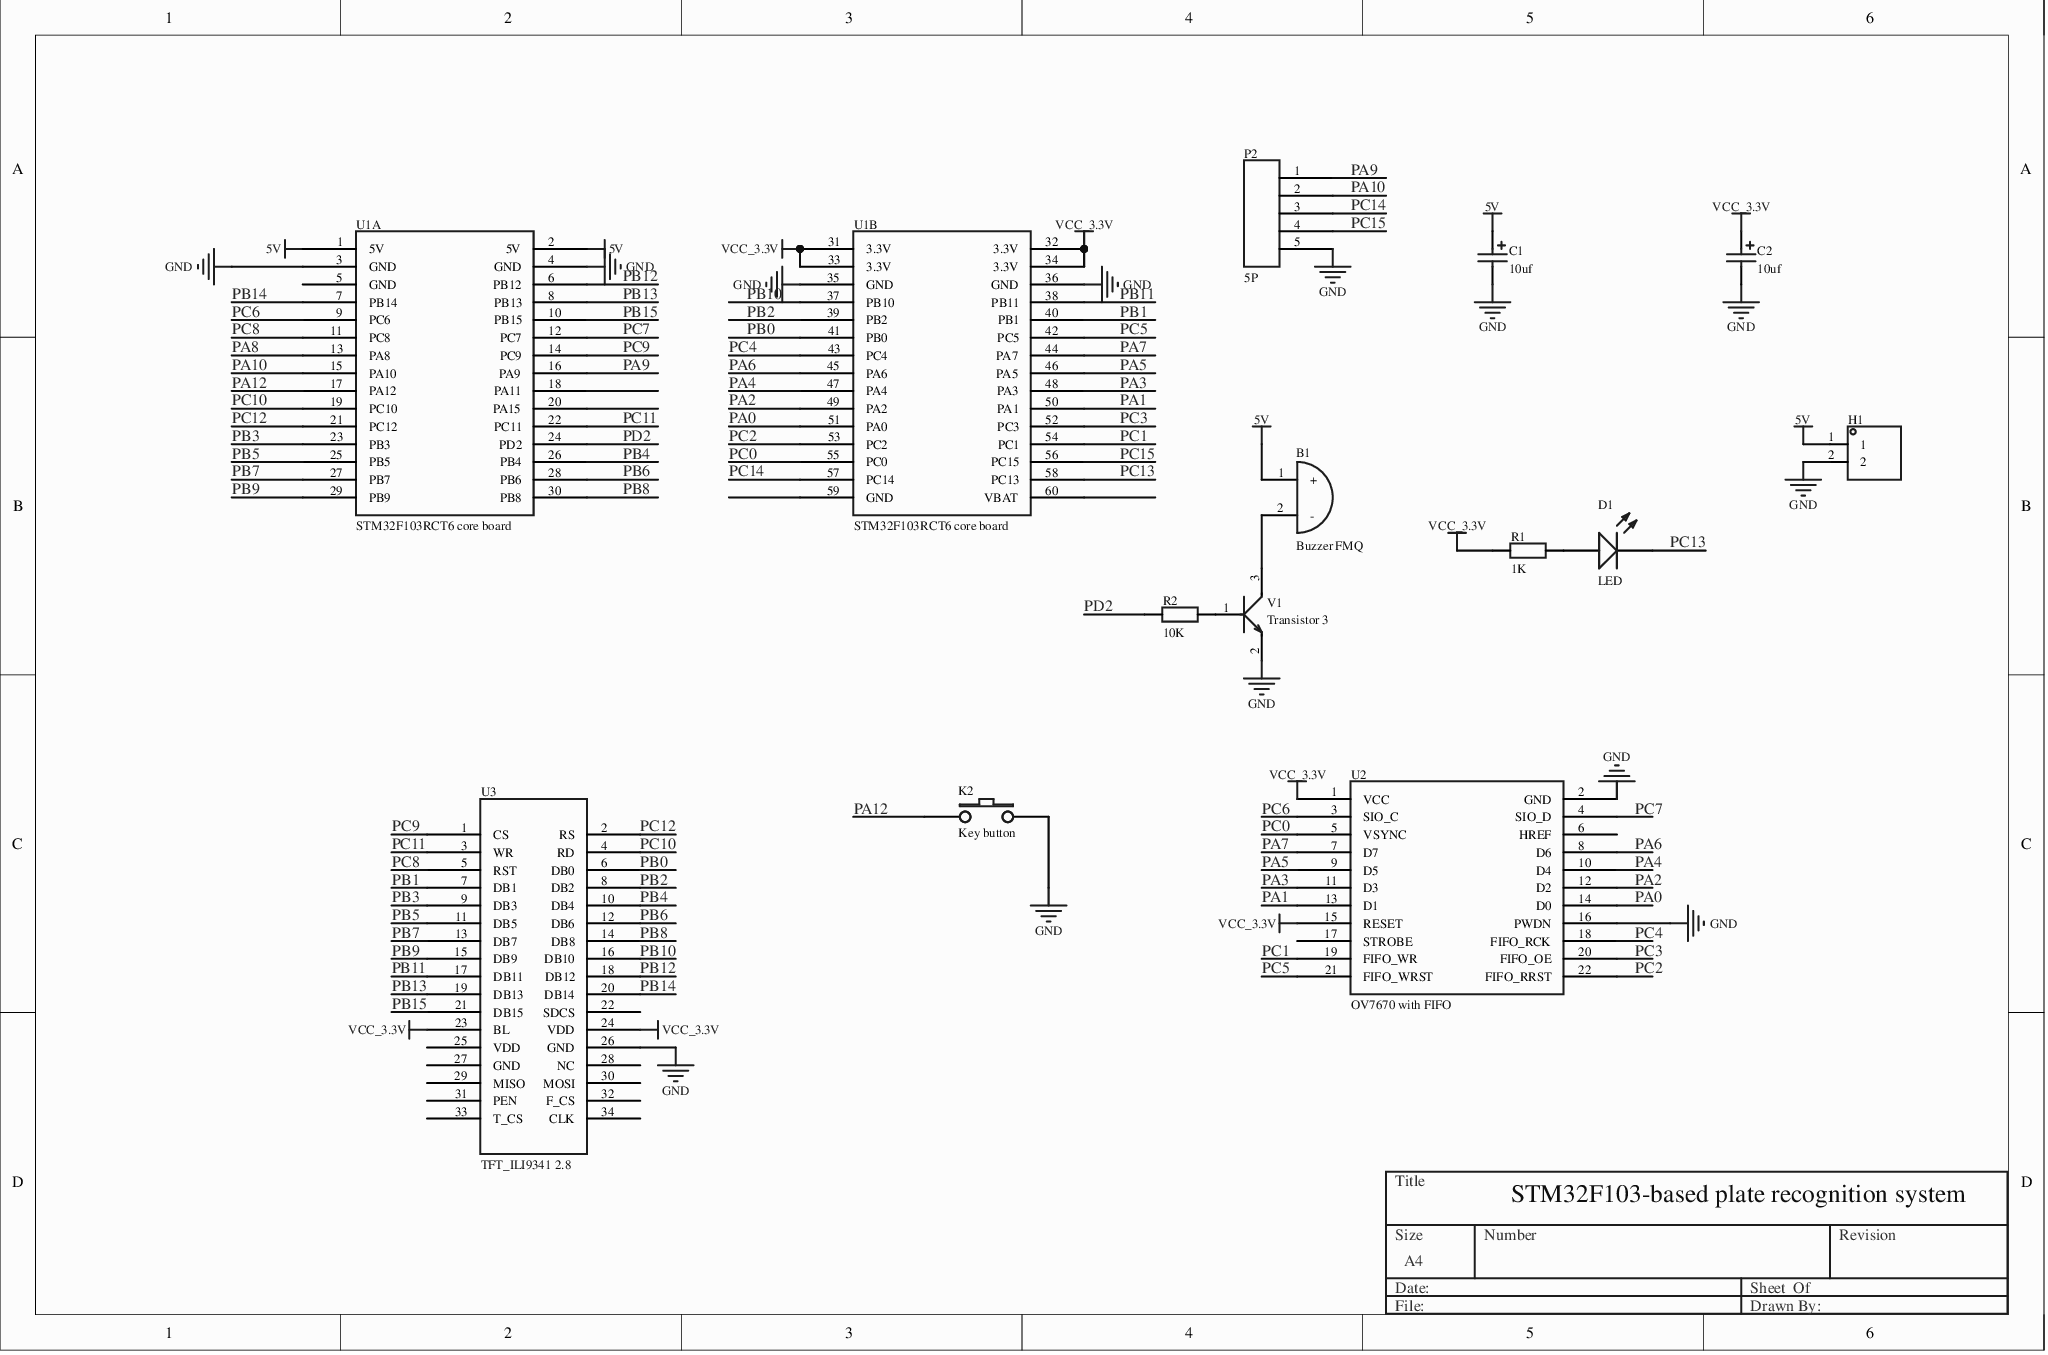
[diagram p0: MISC89050-3.schdoc]
# Altium project MISC89050.PrjPcb
1 sheet, 13 parts. Net scope: global (net labels, ports and power ports of the same name join across sheets).
Board file: MISC89050.pcbdoc

## Sheet MISC89050-3.schdoc
size 292 x 193 mm; @Page No: 1; @Page Count: 1; @Schematic Name: MISC89050; @Project Name: MISC89050; @Board Name: MISC89050; @Update Date: 2025-05-08; @Create Time: 17:11:40; @Update Time: 17:11:44; @Create Date: 2025-05-08

### Parts
B1  Buzzer FMQ  [蜂鸣器]
C1  10uf  [CD0.254cm]
C2  10uf  [CD0.254cm]
D1  LED  [发光二极管FZ]
H1  (no value)  [HDR-TH_2P-P2.54-V-M-1]
K2  Key button  [按键]
P2  5P  [5ZHEN-100mil]
R1  1K  [电阻FZ]
R2  10K  [电阻FZ]
U1  STM32F103RCT6 core board  [STM32F103RC/RB 核心板]  (parts A,B of 2)
U2  OV7670 with FIFO  [OV7670模块]
U3  TFT_ILI9341 2.8  [2.8寸TFT]
V1  Transistor 3  [三极管FZ]

### Nets
5V: B1.1(+) C1.1 H1.1 U1.1(5V) U1.2(5V)
GND: C1.2 C2.2 H1.2 K2.2 P2.5 U1.3(GND) U1.4(GND) U1.35(GND) U1.36(GND) U2.2(GND) U2.16(PWDN) U3.26(GND) V1.2
VCC_3.3V: C2.1 R1.1 U1.31(3.3V) U1.32(3.3V) U1.33(3.3V) U1.34(3.3V) U2.1(VCC) U2.15(RESET) U3.23(BL) U3.24(VDD)
PA0: U1.51(PA0) U2.14(D0)
PA1: U1.50(PA1) U2.13(D1)
PA2: U1.49(PA2) U2.12(D2)
PA3: U1.48(PA3) U2.11(D3)
PA4: U1.47(PA4) U2.10(D4)
PA5: U1.46(PA5) U2.9(D5)
PA6: U1.45(PA6) U2.8(D6)
PA7: U1.44(PA7) U2.7(D7)
PA8: U1.13(PA8)
PA9: P2.1 U1.16(PA9)
PA10: P2.2 U1.15(PA10)
PA12: K2.1 U1.17(PA12)
PB0: U1.41(PB0) U3.6(DB0)
PB1: U1.40(PB1) U3.7(DB1)
PB2: U1.39(PB2) U3.8(DB2)
PB3: U1.23(PB3) U3.9(DB3)
PB4: U1.26(PB4) U3.10(DB4)
PB5: U1.25(PB5) U3.11(DB5)
PB6: U1.28(PB6) U3.12(DB6)
PB7: U1.27(PB7) U3.13(DB7)
PB8: U1.30(PB8) U3.14(DB8)
PB9: U1.29(PB9) U3.15(DB9)
PB10: U1.37(PB10) U3.16(DB10)
PB11: U1.38(PB11) U3.17(DB11)
PB12: U1.6(PB12) U3.18(DB12)
PB13: U1.8(PB13) U3.19(DB13)
PB14: U1.7(PB14) U3.20(DB14)
PB15: U1.10(PB15) U3.21(DB15)
PC0: U1.55(PC0) U2.5(VSYNC)
PC1: U1.54(PC1) U2.19(FIFO_WR)
PC2: U1.53(PC2) U2.22(FIFO_RRST)
PC3: U1.52(PC3) U2.20(FIFO_OE)
PC4: U1.43(PC4) U2.18(FIFO_RCK)
PC5: U1.42(PC5) U2.21(FIFO_WRST)
PC6: U1.9(PC6) U2.3(SIO_C)
PC7: U1.12(PC7) U2.4(SIO_D)
PC8: U1.11(PC8) U3.5(RST)
PC9: U1.14(PC9) U3.1(CS)
PC10: U1.19(PC10) U3.4(RD)
PC11: U1.22(PC11) U3.3(WR)
PC12: U1.21(PC12) U3.2(RS)
PC13: D1.2(K) U1.58(PC13)
PC14: P2.3 U1.57(PC14)
PC15: P2.4 U1.56(PC15)
PD2: R2.1 U1.24(PD2)
NetB1_2: B1.2(-) V1.3
NetD1_1: D1.1(A) R1.2
NetR2_2: R2.2 V1.1

Not connected (* = marked no-connect by the designer): U1 5(GND) 18(PA11) 20(PA15) 59(GND) 60(VBAT); U2 6(HREF) 17(STROBE); U3 22(SDCS) 25(VDD) 27(GND) 28(NC) 29(MISO) 30(MOSI) 31(PEN) 32(F_CS) 33(T_CS) 34(CLK)

### Notes on the sheet
- STM32F103-based plate recognition system
- Title
- File:
- Date:
- Size
- A4
- Number
- Drawn By:
- Sheet
- Of
- Revision

### Library data of the parts
B1 = 蜂鸣器FMQ: AddInBom: yes; Origin Footprint: Buzzer; Device: Buzzer FMQ; Symbol: Buzzer FMQ; Design Item ID: Buzzer FMQ; Library Name: Microcontroller 1; FootprintName: Buzzer; ConvertToPcb: yes
C1 C2 = 10uf: Symbol: Electrolytic capacitor; AddInBom: yes; Origin Footprint: CD0.254cm; Device: 10uf; Design Item ID: Electrolytic capacitor; Library Name: Microcontroller 1; FootprintName: CD0.254cm; ConvertToPcb: yes
D1 = 发光二级管: Origin Footprint: LED FZ; AddInBom: yes; Device: LED; Symbol: LED; Design Item ID: LED; Library Name: Microcontroller 1; FootprintName: LED FZ; ConvertToPcb: yes
H1 = HDR-M_2.54_1x2P: Symbol: 210S-1*2P L=11.6MMGold-plated black; ConvertToPcb: yes; ModelId: 79b2e9f2d70a4d68a1b7098f27c6d4c5; ModelName: HDR-M-2.54_1x2; ModelTransform: 200,100,0,0,0,0,0,0,-118.11; Device: HDR-M_2.54_1x2P; AddInBom: yes; SupplierPart: C124375; Supplier Footprint: 插件; FootprintName: HDR-TH_2P-P2.54-V-M-1
K2 = key按键: AddInBom: yes; Origin Footprint: Button; Device: Key button; Symbol: Key button; Design Item ID: Key button; Library Name: Microcontroller 1; FootprintName: Button; ConvertToPcb: yes
P2 = 5P: AddInBom: yes; Origin Footprint: 5ZHEN-100mil; Device: 5P; Symbol: 5P; Design Item ID: 5P; Library Name: Assorted connectors; FootprintName: 5ZHEN-100mil; ConvertToPcb: yes
R1 = 1K: Origin Footprint: Resistor FZ; Symbol: Resistor R; AddInBom: yes; Device: 1K; Design Item ID: Resistor R; Library Name: Microcontroller 1; FootprintName: Resistor FZ; ConvertToPcb: yes
R2 = 10K: Origin Footprint: Resistor FZ; Symbol: Resistor R; AddInBom: yes; Device: 10K; Design Item ID: Resistor R; Library Name: Microcontroller 1; FootprintName: Resistor FZ; ConvertToPcb: yes
U1 = STM32F103RCT6核心板: Origin Footprint: STM32F103RC/RB core board; AddInBom: yes; Device: STM32F103RCT6 core board; Symbol: STM32F103RCT6 core board; Design Item ID: STM32F103RCT6 core board; Library Name: Microcontroller 1; FootprintName: STM32F103RC/RB core board; ConvertToPcb: yes
U2 = OV7670 with FIFO: FIFO; Origin Footprint: OV7670 module; AddInBom: yes; Device: OV7670 with FIFO; Symbol: OV7670; Design Item ID: OV7670; Library Name: OV7670 camera module; LatestRevisionDate: 17-Jul-2002; LatestRevisionNote: Re-released for DXP Platform.; FootprintName: OV7670 module; ConvertToPcb: yes; Publisher: Altium Limited
U3 = TFT_ILI9341 2.8: ILI9341; Origin Footprint: 2.8-inch TFT; Symbol: TFT; AddInBom: yes; Device: TFT_ILI9341 2.8; Design Item ID: TFT; Library Name: ILI9341 color screen; LatestRevisionDate: 17-Jul-2002; LatestRevisionNote: Re-released for DXP Platform.; FootprintName: 2.8-inch TFT; ConvertToPcb: yes; Publisher: Altium Limited
V1 = 三极管3: Origin Footprint: Transistor FZ; AddInBom: yes; Device: Transistor 3; Symbol: Transistor 3; Design Item ID: Transistor 3; Library Name: Microcontroller 1; FootprintName: Transistor FZ; ConvertToPcb: yes